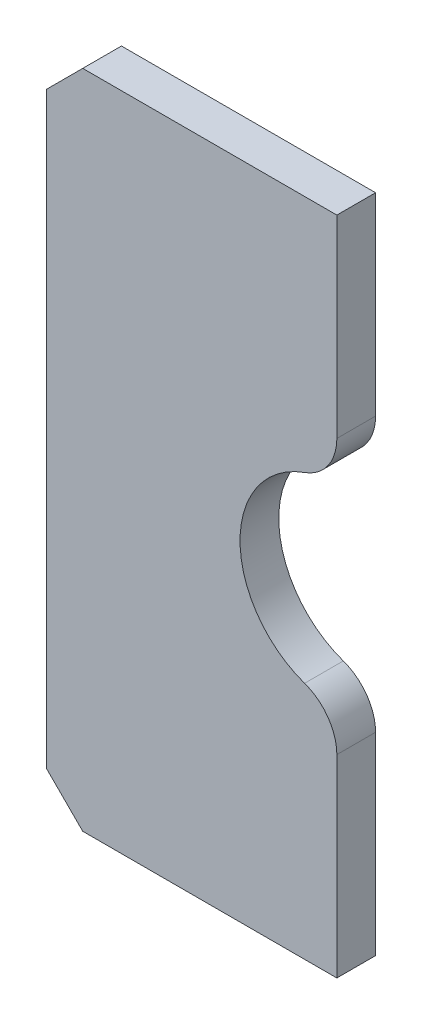
from build123d import *

# Parameters (mm, degrees)
BOSS_EXTRUDE1_DEPTH = 16


with BuildPart() as part:
    # Sketch1 → Boss-Extrude1 (new body)
    with BuildSketch(Plane.XY):
        with BuildLine():
            Line((0, 258), (15, 273))
            Line((15, 273), (120, 273))
            Line((120, 273), (120, 193.068542495))
            ThreePointArc((120, 193.068542495), (116.329931619, 181.521537111), (106.666666667, 174.212361663))
            ThreePointArc((106.666666667, 174.212361663), (80, 136.5), (106.666666667, 98.787638337))
            ThreePointArc((106.666666667, 98.787638337), (116.329931619, 91.478462889), (120, 79.931457505))
            Line((120, 79.931457505), (120, 0))
            Line((120, 0), (15, 0))
            Line((15, 0), (0, 15))
            Line((0, 15), (0, 258))
        make_face()
    extrude(amount=BOSS_EXTRUDE1_DEPTH)


solid = part.part
